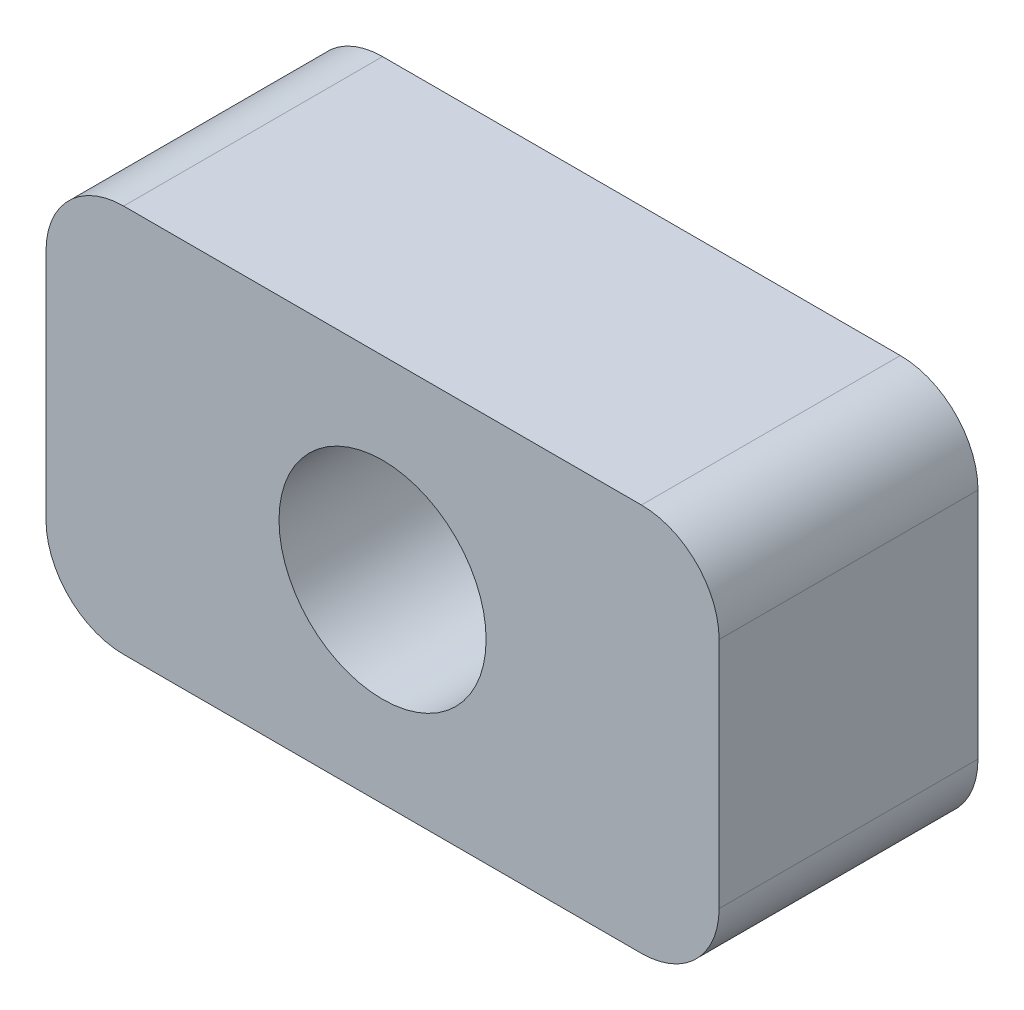
from build123d import *

# Parameters (mm, degrees)
SKETCH1_W           = 26
SKETCH1_H           = 15
SKETCH1_R           = 4
BOSS_EXTRUDE1_DEPTH = 10
FILLET1_R           = 3


with BuildPart() as part:
    # Sketch1 → Boss-Extrude1 (new body)
    with BuildSketch(Plane.XY):
        Rectangle(SKETCH1_W, SKETCH1_H)
        Circle(SKETCH1_R, mode=Mode.SUBTRACT)
    extrude(amount=BOSS_EXTRUDE1_DEPTH)

    # Fillet1
    fillet1_edges = [part.edges().sort_by_distance(p)[0] for p in [
        (13, -7.5, 5),
        (-13, -7.5, 5),
        (-13, 7.5, 5),
        (13, 7.5, 5),
    ]]
    fillet(fillet1_edges, radius=FILLET1_R)


solid = part.part
